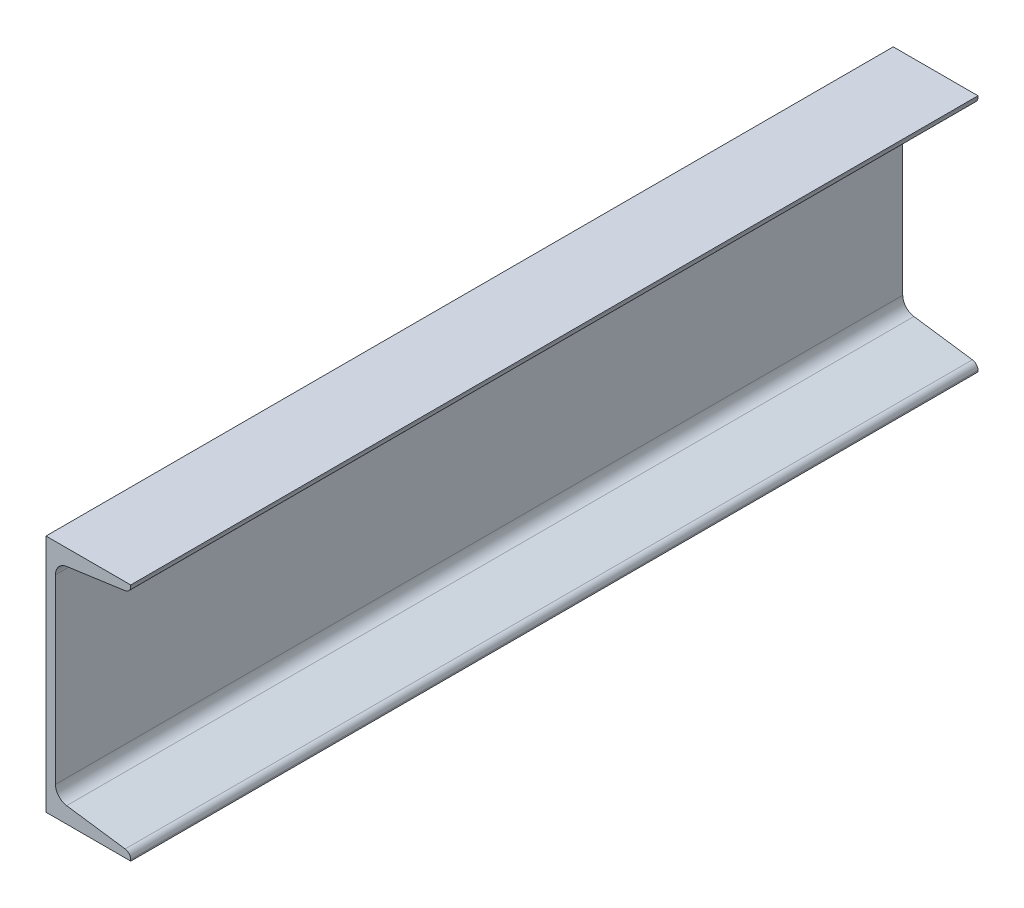
SolidWorks part; units mm, degrees
material "1023 碳钢板 (SS)"
ref_plane "前视基准面" through (0, 0, 0) normal (0, 0, 1) x (1, 0, 0)
ref_plane "上视基准面" through (0, 0, 0) normal (0, 1, 0) x (1, 0, 0)
ref_plane "右视基准面" through (0, 0, 0) normal (1, 0, 0) x (0, 0, -1)
sketch "草图1" plane through (0, 0, 0) normal (0, 0, 1) x (1, 0, 0)
  line L0 (0, 0) -> (-85, 0)
  line L1 (-85, 0) -> (-85, -240)
  line L2 (-85, -240) -> (0, -240)
  line L3 (0, -240) -> (0, -238.6233)
  line L4 (-5.5954, -232.1866) -> (-64.3093, -223.9349)
  line L5 (-75.5, -211.0614) -> (-75.5, -28.9386)
  line L6 (-64.3093, -16.0651) -> (-5.5954, -7.8134)
  line L7 (0, -1.3767) -> (0, 0)
  line L8 (-42.5, -227) -> (-42.5, -240) construction
  arc A0 (-64.3093, -223.9349) -> (-75.5, -211.0614) centre (-62.5, -211.0614) cw
  arc A1 (-75.5, -28.9386) -> (-64.3093, -16.0651) centre (-62.5, -28.9386) cw
  arc A2 (0, -238.6233) -> (-5.5954, -232.1866) centre (-6.5, -238.6233) ccw
  arc A3 (-5.5954, -7.8134) -> (0, -1.3767) centre (-6.5, -1.3767) ccw
  dimension "D7" = 13
  dimension "D8" = 6.5
  dimension "D1" = 240
  dimension "D2" = 85
  dimension "D3" = 42.5
  dimension "D4" = 13
  dimension "D5" = 9.5
  dimension "D6" = 8
extrude "凸台-拉伸1" add sketch "草图1" along normal blind 850 contours A3 L6 A1 L5 A0 L4 A2 L3 L2 L1 L0 L7
sketch "草图2" plane through (-85, 0, 0) normal (-1, 0, 0) x (0, 0, 1)
  line L0 (850, 0) -> (0, 0) construction
  line L2 (0, -211.0614) -> (0, -28.9386) construction
  circle A0 centre (2840, -126) radius 10
  circle A1 centre (2840, -196) radius 10
  circle A2 centre (2640, -126) radius 10
  circle A3 centre (2640, -196) radius 10
  circle A4 centre (2440, -126) radius 10
  circle A5 centre (2440, -196) radius 10
  circle A6 centre (2240, -126) radius 10
  circle A7 centre (2240, -196) radius 10
  circle A8 centre (2040, -126) radius 10
  circle A9 centre (2040, -196) radius 10
  circle A10 centre (1840, -126) radius 10
  circle A11 centre (1840, -196) radius 10
  circle A12 centre (1640, -126) radius 10
  circle A13 centre (1640, -196) radius 10
  circle A14 centre (1440, -126) radius 10
  circle A15 centre (1440, -196) radius 10
  circle A16 centre (1240, -126) radius 10
  circle A17 centre (1240, -196) radius 10
  circle A18 centre (1040, -126) radius 10
  circle A19 centre (1040, -196) radius 10
  circle A20 centre (840, -126) radius 10
  circle A21 centre (840, -196) radius 10
  circle A22 centre (640, -126) radius 10
  circle A23 centre (640, -196) radius 10
  circle A24 centre (440, -126) radius 10
  circle A25 centre (440, -196) radius 10
  circle A26 centre (240, -126) radius 10
  circle A27 centre (240, -196) radius 10
  dimension "D3" = 240
  dimension "D4" = 20
  dimension "D1" = 70
  dimension "D2" = 126
  dimension "D5" = 14
